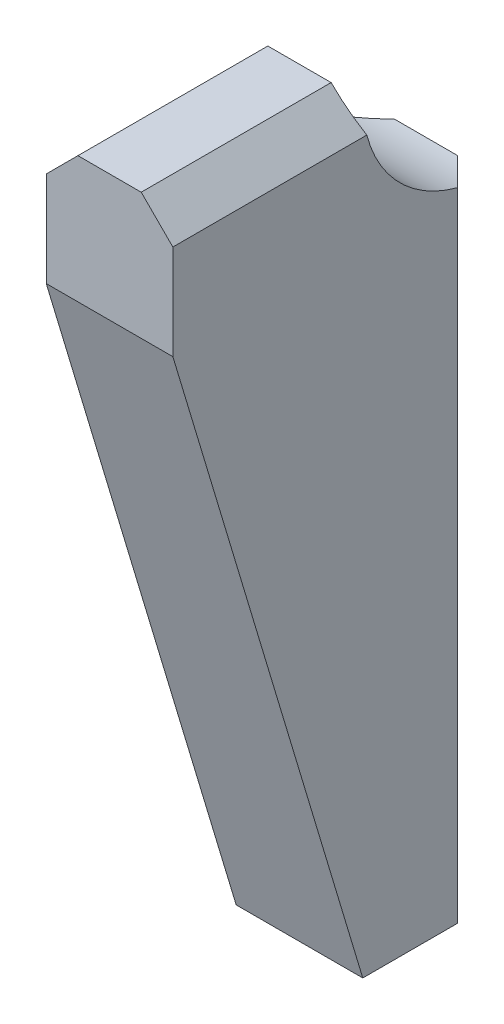
SolidWorks part; units mm, degrees
material "Q235-A"
ref_plane "Front Plane" through (0, 0, 0) normal (0, 0, 1) x (1, 0, 0)
ref_plane "Top Plane" through (0, 0, 0) normal (0, 1, 0) x (1, 0, 0)
ref_plane "Right Plane" through (0, 0, 0) normal (1, 0, 0) x (0, 0, -1)
sketch "Sketch1" plane through (0, 0, 0) normal (1, 0, 0) x (0, 0, -1)
  line L0 (0, 0) -> (0, 200)
  line L1 (-40, 240) -> (-100, 240)
  line L2 (-100, 240) -> (-100, 200)
  line L3 (-100, 200) -> (-40, 0)
  line L4 (-40, 0) -> (0, 0)
  arc A0 (-40, 240) -> (0, 200) centre (0, 240) ccw
  dimension "D1" = 80
  dimension "D2" = 240
  dimension "D3" = 40
  dimension "D4" = 40
  dimension "D5" = 100
extrude "Boss-Extrude1" add sketch "Sketch1" along normal mid plane 40
chamfer "Chamfer1" distance 10 angle 45 4 edges at (-20, 100, 0) (20, 100, 0) (20, 240, 70) (-20, 240, 70)
